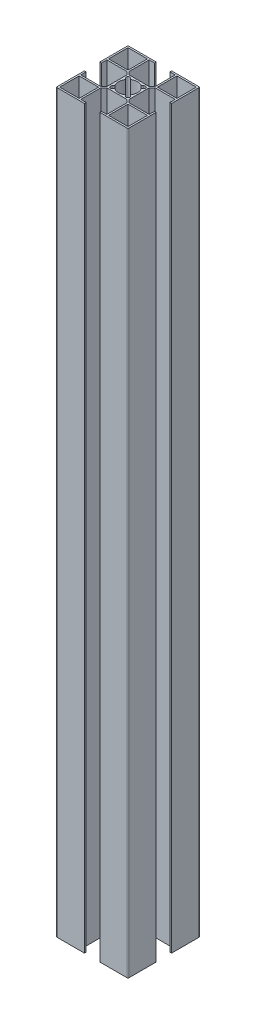
SolidWorks part; units mm, degrees
material "6061 Aluminium alloy"
ref_plane "Front" through (0, 0, 0) normal (0, 0, 1) x (1, 0, 0)
ref_plane "Top" through (0, 0, 0) normal (0, 1, 0) x (1, 0, 0)
ref_plane "Right" through (0, 0, 0) normal (1, 0, 0) x (0, 0, -1)
sketch "Sketch1" plane through (0, 0, 0) normal (0, 1, 0) x (1, 0, 0)
  line L0 (0, 0) -> (0, 20) construction
  line L1 (0, 0) -> (-20, 0) construction
  line L2 (-4.3, 20) -> (-19.5, 20)
  line L3 (-20, 19.5) -> (-20, 4.3)
  line L4 (-20, 4.3) -> (-19.05, 4.3)
  line L5 (-19.05, 4.3) -> (-19.05, 7.25)
  line L6 (-19.05, 7.25) -> (-7.9218, 7.25)
  line L7 (0, 0) -> (-4.3841, 4.3841) construction
  line L8 (-4.3, 20) -> (-4.3, 19.05)
  line L9 (-4.3, 19.05) -> (-7.25, 19.05)
  line L10 (-7.25, 19.05) -> (-7.25, 7.9218)
  line L11 (-7.25, 7.9218) -> (-5.5282, 6.2)
  line L12 (-8.2, 19.05) -> (-19.05, 19.05)
  line L13 (-19.05, 19.05) -> (-19.05, 8.2)
  line L14 (-19.05, 8.2) -> (-8.2, 8.2)
  line L15 (-7.9218, 7.25) -> (-6.2, 5.5282)
  line L16 (-8.2, 19.05) -> (-8.2, 8.2)
  line L17 (-5.5282, 6.2) -> (0, 6.2)
  line L18 (-6.2, 5.5282) -> (-6.2, 0)
  line L19 (-5.0912, 3.677) -> (-4.3875, 2.9732)
  line L20 (-3.677, 5.0912) -> (-2.9732, 4.3875)
  line L21 (0, 6.2) -> (0, 5.3)
  line L22 (-5.3, 0) -> (-6.2, 0)
  arc A0 (-4.3875, 2.9732) -> (-5.3, 0) centre (0, 0) ccw
  arc A1 (-19.5, 20) -> (-20, 19.5) centre (-19.5, 19.5) ccw
  circle A2 centre (0, 0) radius 7.2 construction
  arc A3 (-3.677, 5.0912) -> (-5.0912, 3.677) centre (-4.3841, 4.3841) ccw
  arc A4 (0, 5.3) -> (-2.9732, 4.3875) centre (0, 0) ccw
  dimension "D1" = 10.6
  dimension "D5" = 0.5
  dimension "D17" = 14.4
  dimension "D18" = 2
  dimension "D2" = 40
  dimension "D3" = 40
  dimension "D4" = 8.6
  dimension "D6" = 0.95
  dimension "D7" = 8.6
  dimension "D8" = 14.5
  dimension "D9" = 0.95
  dimension "D10" = 0.95
  dimension "D11" = 0.95
  dimension "D12" = 0.95
  dimension "D13" = 14.5
  dimension "D14" = 13.8
  dimension "D15" = 45
  dimension "D16" = 13.8
extrude "Boss-Extrude1" add sketch "Sketch1" along normal blind 410
mirror "Mirror1" about plane through (0, 0, 0) normal (1, 0, 0) of "Boss-Extrude1"
mirror "Mirror2" about plane through (0, 0, 0) normal (0, 0, 1) of "Mirror1", "Boss-Extrude1"
